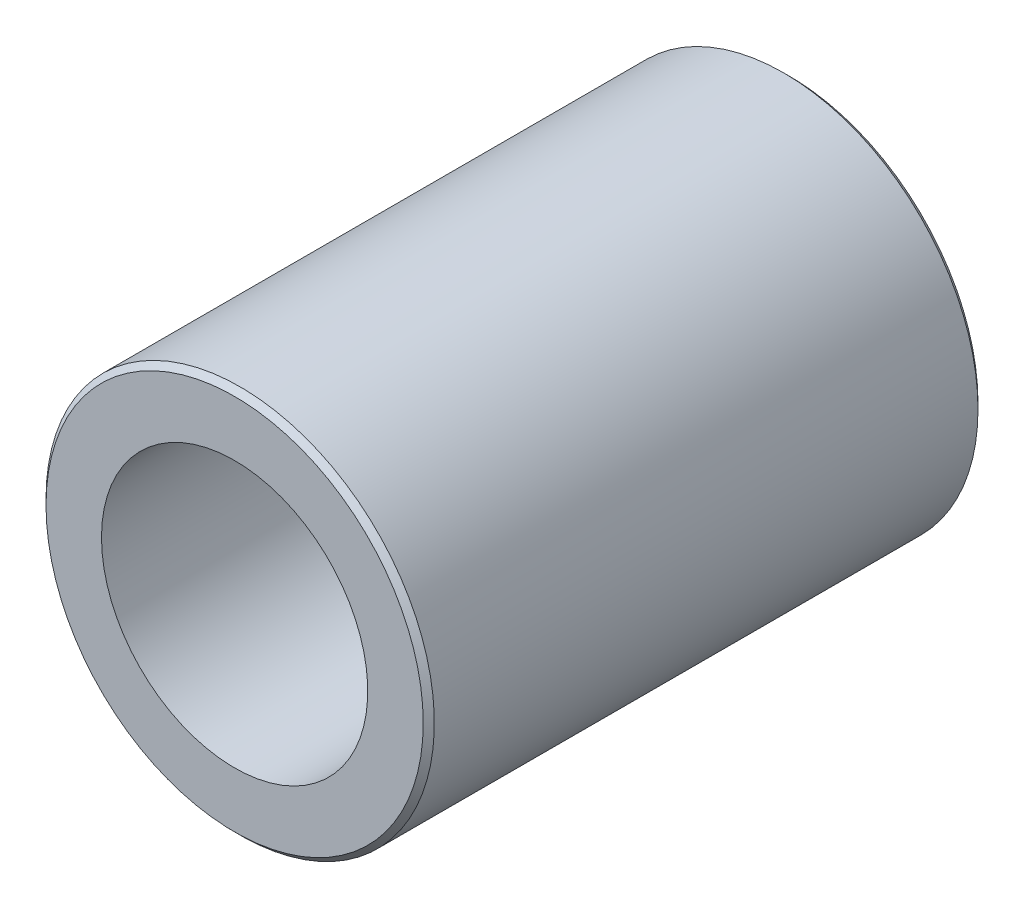
from build123d import *


with BuildPart() as part:
    # Sketch1 → Revolve1 (revolve)
    with BuildSketch(Plane.XZ, mode=Mode.PRIVATE) as revolve1_sk:
        Polygon((12, 28), (12.5, 28), (12.5, 0), (17, 0), (17.5, 0.5), (17.5, 49.5), (17, 50), (12, 50), align=None)
    revolve(revolve1_sk.sketch.rotate(Axis((0, 0, 50), (0, 0, -1)), 180), axis=Axis((0, 0, 50), (0, 0, -1)))


solid = part.part
